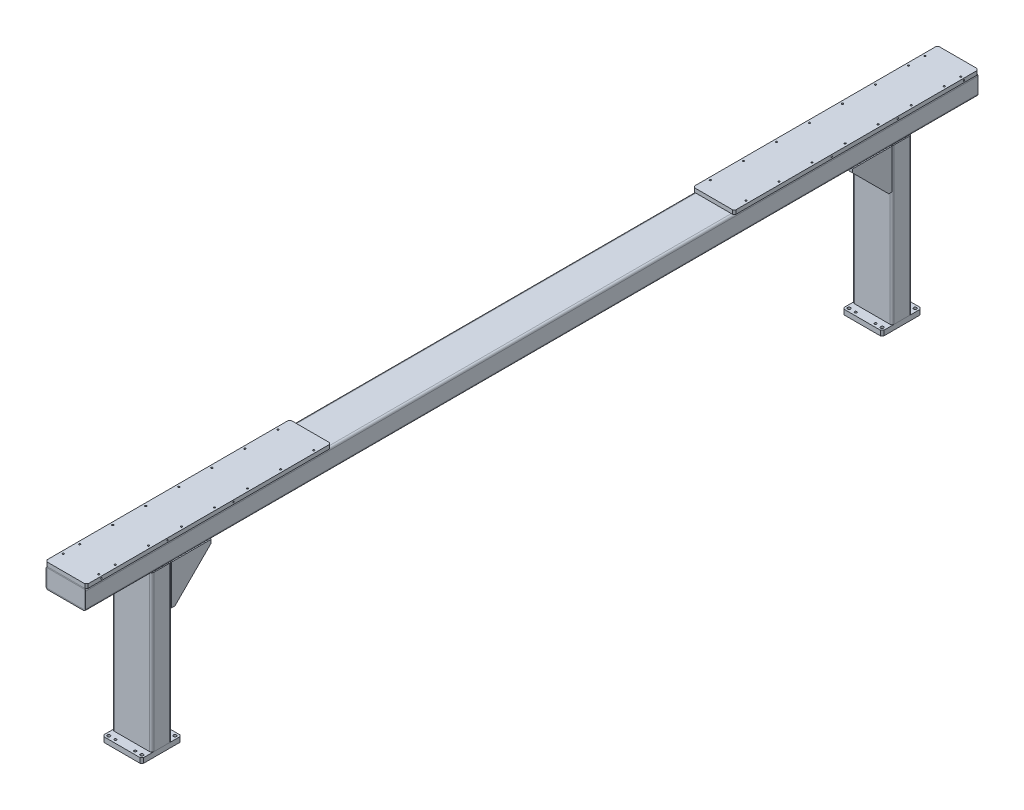
from build123d import *

# Parameters (mm, degrees)
F_120_X_60_X_3_2_1_DEPTH       = 500
F_120_X_60_X_3_2_1_2_DEPTH     = 500
F_120_X_60_X_3_2_2_DEPTH       = 2700
SKETCH_4_W                     = 125
SKETCH_4_H                     = 740
EXTRUDE_1_DEPTH                = 12
SKETCH_5_W                     = 120
SKETCH_5_H                     = 120
EXTRUDE_2_DEPTH                = 15
EXTRUDE_2_2_DEPTH              = 15
HOLE_WIZARD_9_0_9_1_AT_2_COUNT = 2
HOLE_WIZARD_9_0_9_1_AT_2_PITCH = 100
HOLE_WIZARD_9_0_9_1_AT_3_COUNT = 2
HOLE_WIZARD_9_0_9_1_AT_3_PITCH = 141.421356237
HOLE_WIZARD_9_0_9_1_AT_4_COUNT = 2
HOLE_WIZARD_9_0_9_1_AT_4_PITCH = 100
HOLE_WIZARD_9_0_9_1_AT_5_COUNT = 2
HOLE_WIZARD_9_0_9_1_AT_5_PITCH = 2342.135777448
HOLE_WIZARD_9_0_9_1_AT_6_COUNT = 2
HOLE_WIZARD_9_0_9_1_AT_6_PITCH = 2242.231031807
HOLE_WIZARD_9_0_9_1_AT_7_COUNT = 2
HOLE_WIZARD_9_0_9_1_AT_7_PITCH = 2240
HOLE_WIZARD_9_0_9_1_AT_8_COUNT = 2
HOLE_WIZARD_9_0_9_1_AT_8_PITCH = 2340
HOLE_WIZARD_M8_1_AT_2_COUNT    = 2
HOLE_WIZARD_M8_1_AT_2_PITCH    = 100
HOLE_WIZARD_M8_1_AT_3_COUNT    = 2
HOLE_WIZARD_M8_1_AT_3_PITCH    = 116.619037897
HOLE_WIZARD_M8_1_AT_4_COUNT    = 2
HOLE_WIZARD_M8_1_AT_4_PITCH    = 60
HOLE_WIZARD_M8_1_AT_5_COUNT    = 2
HOLE_WIZARD_M8_1_AT_5_PITCH    = 2140.84095626
HOLE_WIZARD_M8_1_AT_6_COUNT    = 2
HOLE_WIZARD_M8_1_AT_6_PITCH    = 2240.803427345
HOLE_WIZARD_M8_1_AT_7_COUNT    = 2
HOLE_WIZARD_M8_1_AT_7_PITCH    = 2240
HOLE_WIZARD_M8_1_AT_8_COUNT    = 2
HOLE_WIZARD_M8_1_AT_8_PITCH    = 2140
CHAMFER_1_SIZE                 = 5
HOLE_WIZARD_M6_1_AT_2_COUNT    = 2
HOLE_WIZARD_M6_1_AT_2_PITCH    = 108
HOLE_WIZARD_M6_1_AT_3_COUNT    = 2
HOLE_WIZARD_M6_1_AT_3_PITCH    = 147.186955944
HOLE_WIZARD_M6_1_AT_4_COUNT    = 2
HOLE_WIZARD_M6_1_AT_4_PITCH    = 227.297162323
HOLE_WIZARD_M6_1_AT_5_COUNT    = 2
HOLE_WIZARD_M6_1_AT_5_PITCH    = 318.847926134
HOLE_WIZARD_M6_1_AT_6_COUNT    = 2
HOLE_WIZARD_M6_1_AT_6_PITCH    = 414.323545071
HOLE_WIZARD_M6_1_AT_7_COUNT    = 2
HOLE_WIZARD_M6_1_AT_7_PITCH    = 511.531035227
HOLE_WIZARD_M6_1_AT_8_COUNT    = 2
HOLE_WIZARD_M6_1_AT_8_PITCH    = 100
HOLE_WIZARD_M6_1_AT_9_COUNT    = 2
HOLE_WIZARD_M6_1_AT_9_PITCH    = 200
HOLE_WIZARD_M6_1_AT_10_COUNT   = 2
HOLE_WIZARD_M6_1_AT_10_PITCH   = 300
HOLE_WIZARD_M6_1_AT_11_COUNT   = 2
HOLE_WIZARD_M6_1_AT_11_PITCH   = 400
HOLE_WIZARD_M6_1_AT_12_COUNT   = 2
HOLE_WIZARD_M6_1_AT_12_PITCH   = 500
HOLE_WIZARD_M6_1_AT_13_COUNT   = 2
HOLE_WIZARD_M6_1_AT_13_PITCH   = 650
HOLE_WIZARD_M6_1_AT_14_COUNT   = 2
HOLE_WIZARD_M6_1_AT_14_PITCH   = 658.911223155
HOLE_WIZARD_M6_1_AT_15_COUNT   = 2
HOLE_WIZARD_M6_1_AT_15_PITCH   = 600
HOLE_WIZARD_M6_1_AT_16_COUNT   = 2
HOLE_WIZARD_M6_1_AT_16_PITCH   = 609.642518202
CHAMFER_3_SIZE                 = 5
HOLE_WIZARD_M5_1_AT_2_COUNT    = 2
HOLE_WIZARD_M5_1_AT_2_PITCH    = 200
HOLE_WIZARD_M5_1_AT_3_COUNT    = 2
HOLE_WIZARD_M5_1_AT_3_PITCH    = 400
CHAMFER_4_SIZE                 = 5
SKETCH_32_W                    = 700
SKETCH_32_H                    = 15
EXTRUDE_3_DEPTH                = 7
EXTRUDE_3_2_DEPTH              = 7
HOLE_WIZARD_M4_3_AT_2_COUNT    = 2
HOLE_WIZARD_M4_3_AT_2_PITCH    = 60
HOLE_WIZARD_M4_3_AT_3_COUNT    = 2
HOLE_WIZARD_M4_3_AT_3_PITCH    = 120
HOLE_WIZARD_M4_3_AT_4_COUNT    = 2
HOLE_WIZARD_M4_3_AT_4_PITCH    = 180
HOLE_WIZARD_M4_3_AT_5_COUNT    = 2
HOLE_WIZARD_M4_3_AT_5_PITCH    = 240
HOLE_WIZARD_M4_3_AT_6_COUNT    = 2
HOLE_WIZARD_M4_3_AT_6_PITCH    = 300
HOLE_WIZARD_M4_3_AT_7_COUNT    = 2
HOLE_WIZARD_M4_3_AT_7_PITCH    = 360
HOLE_WIZARD_M4_3_AT_8_COUNT    = 2
HOLE_WIZARD_M4_3_AT_8_PITCH    = 420
HOLE_WIZARD_M4_3_AT_9_COUNT    = 2
HOLE_WIZARD_M4_3_AT_9_PITCH    = 480
HOLE_WIZARD_M4_3_AT_10_COUNT   = 2
HOLE_WIZARD_M4_3_AT_10_PITCH   = 540
HOLE_WIZARD_M4_3_AT_11_COUNT   = 2
HOLE_WIZARD_M4_3_AT_11_PITCH   = 600
HOLE_WIZARD_M4_3_AT_12_COUNT   = 2
HOLE_WIZARD_M4_3_AT_12_PITCH   = 660
HOLE_WIZARD_M4_3_AT_13_COUNT   = 2
HOLE_WIZARD_M4_3_AT_13_PITCH   = 1960
HOLE_WIZARD_M4_3_AT_14_COUNT   = 2
HOLE_WIZARD_M4_3_AT_14_PITCH   = 2020
HOLE_WIZARD_M4_3_AT_15_COUNT   = 2
HOLE_WIZARD_M4_3_AT_15_PITCH   = 2080
HOLE_WIZARD_M4_3_AT_16_COUNT   = 2
HOLE_WIZARD_M4_3_AT_16_PITCH   = 2140
HOLE_WIZARD_M4_3_AT_17_COUNT   = 2
HOLE_WIZARD_M4_3_AT_17_PITCH   = 2200
HOLE_WIZARD_M4_3_AT_18_COUNT   = 2
HOLE_WIZARD_M4_3_AT_18_PITCH   = 2260
HOLE_WIZARD_M4_3_AT_19_COUNT   = 2
HOLE_WIZARD_M4_3_AT_19_PITCH   = 2320
HOLE_WIZARD_M4_3_AT_20_COUNT   = 2
HOLE_WIZARD_M4_3_AT_20_PITCH   = 2380
HOLE_WIZARD_M4_3_AT_21_COUNT   = 2
HOLE_WIZARD_M4_3_AT_21_PITCH   = 2440
HOLE_WIZARD_M4_3_AT_22_COUNT   = 2
HOLE_WIZARD_M4_3_AT_22_PITCH   = 2500
HOLE_WIZARD_M4_3_AT_23_COUNT   = 2
HOLE_WIZARD_M4_3_AT_23_PITCH   = 2560
HOLE_WIZARD_M4_3_AT_24_COUNT   = 2
HOLE_WIZARD_M4_3_AT_24_PITCH   = 2620
HOLE_WIZARD_M4_4_AT_2_COUNT    = 2
HOLE_WIZARD_M4_4_AT_2_PITCH    = 690
HOLE_WIZARD_M4_4_AT_3_COUNT    = 2
HOLE_WIZARD_M4_4_AT_3_PITCH    = 1960
HOLE_WIZARD_M4_4_AT_4_COUNT    = 2
HOLE_WIZARD_M4_4_AT_4_PITCH    = 2650
EXTRUDE_4_DEPTH                = 5
EXTRUDE_5_DEPTH                = 10


with BuildPart() as part:
    # Sketch12 → 矩型管 120 X 60 X 3.2(1) (new body)
    with BuildSketch(Plane(origin=(0, 500, -1120), x_dir=(0, 0, -1), z_dir=(0, -1, 0))):
        with BuildLine():
            Line((-23.6, -60), (23.6, -60))
            ThreePointArc((23.6, -60), (28.1254834, -58.1254834), (30, -53.6))
            Line((30, -53.6), (30, 53.6))
            ThreePointArc((30, 53.6), (28.1254834, 58.1254834), (23.6, 60))
            Line((23.6, 60), (-23.6, 60))
            ThreePointArc((-23.6, 60), (-28.1254834, 58.1254834), (-30, 53.6))
            Line((-30, 53.6), (-30, -53.6))
            ThreePointArc((-30, -53.6), (-28.1254834, -58.1254834), (-23.6, -60))
        make_face()
        with BuildLine():
            Line((-23.6, -56.8), (23.6, -56.8))
            ThreePointArc((23.6, -56.8), (25.8627417, -55.8627417), (26.8, -53.6))
            Line((26.8, -53.6), (26.8, 53.6))
            ThreePointArc((26.8, 53.6), (25.8627417, 55.8627417), (23.6, 56.8))
            Line((23.6, 56.8), (-23.6, 56.8))
            ThreePointArc((-23.6, 56.8), (-25.8627417, 55.8627417), (-26.8, 53.6))
            Line((-26.8, 53.6), (-26.8, -53.6))
            ThreePointArc((-26.8, -53.6), (-25.8627417, -55.8627417), (-23.6, -56.8))
        make_face(mode=Mode.SUBTRACT)
    extrude(amount=F_120_X_60_X_3_2_1_DEPTH)

    # Weld Trim 1
    split(bisect_by=Plane.XZ.offset(-470), keep=Keep.TOP)


with BuildPart() as body_2:
    # Sketch12 on segment 2 (carried to segment 2) → 120 X 60 X 3.2_1 2 (new body)
    with BuildSketch(Plane(origin=(0, 500, 1120), x_dir=(0, 0, -1), z_dir=(0, -1, 0))):
        with BuildLine():
            Line((-23.6, -60), (23.6, -60))
            ThreePointArc((23.6, -60), (28.1254834, -58.1254834), (30, -53.6))
            Line((30, -53.6), (30, 53.6))
            ThreePointArc((30, 53.6), (28.1254834, 58.1254834), (23.6, 60))
            Line((23.6, 60), (-23.6, 60))
            ThreePointArc((-23.6, 60), (-28.1254834, 58.1254834), (-30, 53.6))
            Line((-30, 53.6), (-30, -53.6))
            ThreePointArc((-30, -53.6), (-28.1254834, -58.1254834), (-23.6, -60))
        make_face()
        with BuildLine():
            Line((-23.6, -56.8), (23.6, -56.8))
            ThreePointArc((23.6, -56.8), (25.8627417, -55.8627417), (26.8, -53.6))
            Line((26.8, -53.6), (26.8, 53.6))
            ThreePointArc((26.8, 53.6), (25.8627417, 55.8627417), (23.6, 56.8))
            Line((23.6, 56.8), (-23.6, 56.8))
            ThreePointArc((-23.6, 56.8), (-25.8627417, 55.8627417), (-26.8, 53.6))
            Line((-26.8, 53.6), (-26.8, -53.6))
            ThreePointArc((-26.8, -53.6), (-25.8627417, -55.8627417), (-23.6, -56.8))
        make_face(mode=Mode.SUBTRACT)
    extrude(amount=F_120_X_60_X_3_2_1_2_DEPTH)

    # Weld Trim 1
    split(bisect_by=Plane.XZ.offset(-470), keep=Keep.TOP)


with BuildPart() as body_3:
    # Sketch1 → 矩型管 120 X 60 X 3.2(2) (new body)
    with BuildSketch(Plane(origin=(0, 500, 1350), x_dir=(0, 1, 0), z_dir=(0, 0, -1))):
        with BuildLine():
            Line((-23.6, -60), (23.6, -60))
            ThreePointArc((23.6, -60), (28.1254834, -58.1254834), (30, -53.6))
            Line((30, -53.6), (30, 53.6))
            ThreePointArc((30, 53.6), (28.1254834, 58.1254834), (23.6, 60))
            Line((23.6, 60), (-23.6, 60))
            ThreePointArc((-23.6, 60), (-28.1254834, 58.1254834), (-30, 53.6))
            Line((-30, 53.6), (-30, -53.6))
            ThreePointArc((-30, -53.6), (-28.1254834, -58.1254834), (-23.6, -60))
        make_face()
        with BuildLine():
            Line((-23.6, -56.8), (23.6, -56.8))
            ThreePointArc((23.6, -56.8), (25.8627417, -55.8627417), (26.8, -53.6))
            Line((26.8, -53.6), (26.8, 53.6))
            ThreePointArc((26.8, 53.6), (25.8627417, 55.8627417), (23.6, 56.8))
            Line((23.6, 56.8), (-23.6, 56.8))
            ThreePointArc((-23.6, 56.8), (-25.8627417, 55.8627417), (-26.8, 53.6))
            Line((-26.8, 53.6), (-26.8, -53.6))
            ThreePointArc((-26.8, -53.6), (-25.8627417, -55.8627417), (-23.6, -56.8))
        make_face(mode=Mode.SUBTRACT)
    extrude(amount=F_120_X_60_X_3_2_2_DEPTH)


with BuildPart() as body_4:
    # 草图4 → 凸台-拉伸1 (new body)
    with BuildSketch(Plane(origin=(0, 530, 0), x_dir=(1, 0, 0), z_dir=(0, 1, 0))):
        with Locations((0, 980)):
            Rectangle(SKETCH_4_W, SKETCH_4_H)
    extrude(amount=EXTRUDE_1_DEPTH)

    # 草图25 → M6 螺纹孔1 (revolve, cut)
    with BuildSketch(Plane(origin=(54, 542, -654), x_dir=(0, 0, 1), z_dir=(1, 0, 0))):
        Polygon((0, 0), (0, 16.502151548), (2.5, 15), (2.5, 0), align=None)
    hole_wizard_m6_1 = revolve(axis=Axis((54, 548.35, -654), (0, -1, 0)), mode=Mode.SUBTRACT)

    # M6 螺纹孔1 at 2: M6 螺纹孔1 ×2
    with Locations(*[(-i * HOLE_WIZARD_M6_1_AT_2_PITCH, 0, 0) for i in range(1, HOLE_WIZARD_M6_1_AT_2_COUNT)]):
        add(hole_wizard_m6_1, mode=Mode.SUBTRACT)

    # M6 螺纹孔1 at 3: M6 螺纹孔1 ×2
    with Locations(*[Vector(-0.7337606740181704, 0, -0.679408031498304) * (i * HOLE_WIZARD_M6_1_AT_3_PITCH) for i in range(1, HOLE_WIZARD_M6_1_AT_3_COUNT)]):
        add(hole_wizard_m6_1, mode=Mode.SUBTRACT)

    # M6 螺纹孔1 at 4: M6 螺纹孔1 ×2
    with Locations(*[Vector(-0.47514891473488374, 0, -0.8799053976571926) * (i * HOLE_WIZARD_M6_1_AT_4_PITCH) for i in range(1, HOLE_WIZARD_M6_1_AT_4_COUNT)]):
        add(hole_wizard_m6_1, mode=Mode.SUBTRACT)

    # M6 螺纹孔1 at 5: M6 螺纹孔1 ×2
    with Locations(*[Vector(-0.3387194682727412, 0, -0.940887411868727) * (i * HOLE_WIZARD_M6_1_AT_5_PITCH) for i in range(1, HOLE_WIZARD_M6_1_AT_5_COUNT)]):
        add(hole_wizard_m6_1, mode=Mode.SUBTRACT)

    # M6 螺纹孔1 at 6: M6 螺纹孔1 ×2
    with Locations(*[Vector(-0.26066585229076417, 0, -0.9654290825583873) * (i * HOLE_WIZARD_M6_1_AT_6_PITCH) for i in range(1, HOLE_WIZARD_M6_1_AT_6_COUNT)]):
        add(hole_wizard_m6_1, mode=Mode.SUBTRACT)

    # M6 螺纹孔1 at 7: M6 螺纹孔1 ×2
    with Locations(*[Vector(-0.21113088466305252, 0, -0.9774577993659864) * (i * HOLE_WIZARD_M6_1_AT_7_PITCH) for i in range(1, HOLE_WIZARD_M6_1_AT_7_COUNT)]):
        add(hole_wizard_m6_1, mode=Mode.SUBTRACT)

    # M6 螺纹孔1 at 8: M6 螺纹孔1 ×2
    with Locations(*[(0, 0, -i * HOLE_WIZARD_M6_1_AT_8_PITCH) for i in range(1, HOLE_WIZARD_M6_1_AT_8_COUNT)]):
        add(hole_wizard_m6_1, mode=Mode.SUBTRACT)

    # M6 螺纹孔1 at 9: M6 螺纹孔1 ×2
    with Locations(*[(0, 0, -i * HOLE_WIZARD_M6_1_AT_9_PITCH) for i in range(1, HOLE_WIZARD_M6_1_AT_9_COUNT)]):
        add(hole_wizard_m6_1, mode=Mode.SUBTRACT)

    # M6 螺纹孔1 at 10: M6 螺纹孔1 ×2
    with Locations(*[(0, 0, -i * HOLE_WIZARD_M6_1_AT_10_PITCH) for i in range(1, HOLE_WIZARD_M6_1_AT_10_COUNT)]):
        add(hole_wizard_m6_1, mode=Mode.SUBTRACT)

    # M6 螺纹孔1 at 11: M6 螺纹孔1 ×2
    with Locations(*[(0, 0, -i * HOLE_WIZARD_M6_1_AT_11_PITCH) for i in range(1, HOLE_WIZARD_M6_1_AT_11_COUNT)]):
        add(hole_wizard_m6_1, mode=Mode.SUBTRACT)

    # M6 螺纹孔1 at 12: M6 螺纹孔1 ×2
    with Locations(*[(0, 0, -i * HOLE_WIZARD_M6_1_AT_12_PITCH) for i in range(1, HOLE_WIZARD_M6_1_AT_12_COUNT)]):
        add(hole_wizard_m6_1, mode=Mode.SUBTRACT)

    # M6 螺纹孔1 at 13: M6 螺纹孔1 ×2
    with Locations(*[(0, 0, -i * HOLE_WIZARD_M6_1_AT_13_PITCH) for i in range(1, HOLE_WIZARD_M6_1_AT_13_COUNT)]):
        add(hole_wizard_m6_1, mode=Mode.SUBTRACT)

    # M6 螺纹孔1 at 14: M6 螺纹孔1 ×2
    with Locations(*[Vector(-0.16390675436187938, 0, -0.9864758364372412) * (i * HOLE_WIZARD_M6_1_AT_14_PITCH) for i in range(1, HOLE_WIZARD_M6_1_AT_14_COUNT)]):
        add(hole_wizard_m6_1, mode=Mode.SUBTRACT)

    # M6 螺纹孔1 at 15: M6 螺纹孔1 ×2
    with Locations(*[(0, 0, -i * HOLE_WIZARD_M6_1_AT_15_PITCH) for i in range(1, HOLE_WIZARD_M6_1_AT_15_COUNT)]):
        add(hole_wizard_m6_1, mode=Mode.SUBTRACT)

    # M6 螺纹孔1 at 16: M6 螺纹孔1 ×2
    with Locations(*[Vector(-0.17715299831526468, 0, -0.9841833239736955) * (i * HOLE_WIZARD_M6_1_AT_16_PITCH) for i in range(1, HOLE_WIZARD_M6_1_AT_16_COUNT)]):
        add(hole_wizard_m6_1, mode=Mode.SUBTRACT)

    # 倒角3
    chamfer_3_edges = [body_4.edges().sort_by_distance(p)[0] for p in [
        (-62.5, 536, -610),
        (-62.5, 536, -1350),
        (62.5, 536, -1350),
        (62.5, 536, -610),
    ]]
    chamfer(chamfer_3_edges, length=CHAMFER_3_SIZE)

    # 草图27 → M5 螺纹孔1 (revolve, cut)
    with BuildSketch(Plane(origin=(62.5, 536, -905), x_dir=(0, 0, -1), z_dir=(0, 1, 0))):
        Polygon((0, 0), (0, 13.6618073), (2.1, 12.4), (2.1, 0), align=None)
    hole_wizard_m5_1 = revolve(axis=Axis((68.85, 536, -905), (-1, 0, 0)), mode=Mode.SUBTRACT)

    # M5 螺纹孔1 at 2: M5 螺纹孔1 ×2
    with Locations(*[(0, 0, -i * HOLE_WIZARD_M5_1_AT_2_PITCH) for i in range(1, HOLE_WIZARD_M5_1_AT_2_COUNT)]):
        add(hole_wizard_m5_1, mode=Mode.SUBTRACT)

    # M5 螺纹孔1 at 3: M5 螺纹孔1 ×2
    with Locations(*[(0, 0, -i * HOLE_WIZARD_M5_1_AT_3_PITCH) for i in range(1, HOLE_WIZARD_M5_1_AT_3_COUNT)]):
        add(hole_wizard_m5_1, mode=Mode.SUBTRACT)

    # 镜向1: M5 螺纹孔1 across plane
    add(hole_wizard_m5_1.mirror(Plane(origin=(0, 0, 0), x_dir=(0, 0, 1), z_dir=(1, 0, 0))), mode=Mode.SUBTRACT)

    # 镜向1 copy 1 sketch → 镜向1 copy 1 (revolve, cut)
    with BuildSketch(Plane(origin=(-62.5, 536, -1105), x_dir=(0, 0, -1), z_dir=(0, 1, 0))):
        Polygon((0, 0), (0, -13.6618073), (2.1, -12.4), (2.1, 0), align=None)
    revolve(axis=Axis((-68.85, 536, -1105), (-1, 0, 0)), mode=Mode.SUBTRACT)

    # 镜向1 copy 2 sketch → 镜向1 copy 2 (revolve, cut)
    with BuildSketch(Plane(origin=(-62.5, 536, -1305), x_dir=(0, 0, -1), z_dir=(0, 1, 0))):
        Polygon((0, 0), (0, -13.6618073), (2.1, -12.4), (2.1, 0), align=None)
    revolve(axis=Axis((-68.85, 536, -1305), (-1, 0, 0)), mode=Mode.SUBTRACT)


with BuildPart() as body_5:
    # 草图5 → 凸台-拉伸2 (new body)
    with BuildSketch(Plane.XZ):
        with Locations((0, 1120)):
            Rectangle(SKETCH_5_W, SKETCH_5_H)
    extrude(amount=EXTRUDE_2_DEPTH)


with BuildPart() as body_6:
    # 草图5 → Extrude 2 2 (new body)
    with BuildSketch(Plane.XZ):
        with Locations((0, -1120)):
            Rectangle(SKETCH_5_W, SKETCH_5_H)
    extrude(amount=EXTRUDE_2_2_DEPTH)

    # 草图15 → Ø9.0 (9) 直径孔1 (revolve, cut)
    with BuildSketch(Plane(origin=(-50, -15, -1170), x_dir=(0, 0, -1), z_dir=(1, 0, 0))):
        Polygon((0, 0), (0, 22.703872786), (4.5, 20), (4.5, 0), align=None)
    hole_wizard_9_0_9_1 = revolve(axis=Axis((-50, -21.35, -1170), (0, 1, 0)), mode=Mode.SUBTRACT)

    # Ø9.0 (9) 直径孔1 at 2: Ø9.0 (9) 直径孔1 ×2
    with Locations(*[(0, 0, i * HOLE_WIZARD_9_0_9_1_AT_2_PITCH) for i in range(1, HOLE_WIZARD_9_0_9_1_AT_2_COUNT)]):
        add(hole_wizard_9_0_9_1, mode=Mode.SUBTRACT)

    # Ø9.0 (9) 直径孔1 at 3: Ø9.0 (9) 直径孔1 ×2
    with Locations(*[Vector(0.7071067811865445, 0, 0.7071067811865507) * (i * HOLE_WIZARD_9_0_9_1_AT_3_PITCH) for i in range(1, HOLE_WIZARD_9_0_9_1_AT_3_COUNT)]):
        add(hole_wizard_9_0_9_1, mode=Mode.SUBTRACT)

    # Ø9.0 (9) 直径孔1 at 4: Ø9.0 (9) 直径孔1 ×2
    with Locations(*[(i * HOLE_WIZARD_9_0_9_1_AT_4_PITCH, 0, 0) for i in range(1, HOLE_WIZARD_9_0_9_1_AT_4_COUNT)]):
        add(hole_wizard_9_0_9_1, mode=Mode.SUBTRACT)

    # 草图13 → M8 螺纹孔1 (revolve, cut)
    with BuildSketch(Plane(origin=(-30, 0, -1070), x_dir=(0, 0, 1), z_dir=(1, 0, 0))):
        Polygon((0, 0), (0, 24.292926105), (3.4, 22.25), (3.4, 0), align=None)
    hole_wizard_m8_1 = revolve(axis=Axis((-30, 6.35, -1070), (0, -1, 0)), mode=Mode.SUBTRACT)

    # M8 螺纹孔1 at 2: M8 螺纹孔1 ×2
    with Locations(*[(0, 0, -i * HOLE_WIZARD_M8_1_AT_2_PITCH) for i in range(1, HOLE_WIZARD_M8_1_AT_2_COUNT)]):
        add(hole_wizard_m8_1, mode=Mode.SUBTRACT)

    # M8 螺纹孔1 at 3: M8 螺纹孔1 ×2
    with Locations(*[Vector(0.5144957554275295, 0, -0.8574929257125425) * (i * HOLE_WIZARD_M8_1_AT_3_PITCH) for i in range(1, HOLE_WIZARD_M8_1_AT_3_COUNT)]):
        add(hole_wizard_m8_1, mode=Mode.SUBTRACT)

    # M8 螺纹孔1 at 4: M8 螺纹孔1 ×2
    with Locations(*[(i * HOLE_WIZARD_M8_1_AT_4_PITCH, 0, 0) for i in range(1, HOLE_WIZARD_M8_1_AT_4_COUNT)]):
        add(hole_wizard_m8_1, mode=Mode.SUBTRACT)

    # 倒角4
    chamfer_4_edges = [body_6.edges().sort_by_distance(p)[0] for p in [
        (-60, -7.5, -1180),
        (-60, -7.5, -1060),
        (60, -7.5, -1060),
        (60, -7.5, -1180),
    ]]
    chamfer(chamfer_4_edges, length=CHAMFER_4_SIZE)


with BuildPart() as body_5_1:
    add(body_5.part)

    # Ø9.0 (9) 直径孔1 at 5: Ø9.0 (9) 直径孔1 ×2
    with Locations(*[Vector(0.04269607294457472, 0, 0.9990881069030457) * (i * HOLE_WIZARD_9_0_9_1_AT_5_PITCH) for i in range(1, HOLE_WIZARD_9_0_9_1_AT_5_COUNT)]):
        add(hole_wizard_9_0_9_1, mode=Mode.SUBTRACT)

    # Ø9.0 (9) 直径孔1 at 6: Ø9.0 (9) 直径孔1 ×2
    with Locations(*[Vector(0.044598437262458705, 0, 0.999004994679079) * (i * HOLE_WIZARD_9_0_9_1_AT_6_PITCH) for i in range(1, HOLE_WIZARD_9_0_9_1_AT_6_COUNT)]):
        add(hole_wizard_9_0_9_1, mode=Mode.SUBTRACT)

    # Ø9.0 (9) 直径孔1 at 7: Ø9.0 (9) 直径孔1 ×2
    with Locations(*[(0, 0, i * HOLE_WIZARD_9_0_9_1_AT_7_PITCH) for i in range(1, HOLE_WIZARD_9_0_9_1_AT_7_COUNT)]):
        add(hole_wizard_9_0_9_1, mode=Mode.SUBTRACT)

    # Ø9.0 (9) 直径孔1 at 8: Ø9.0 (9) 直径孔1 ×2
    with Locations(*[(0, 0, i * HOLE_WIZARD_9_0_9_1_AT_8_PITCH) for i in range(1, HOLE_WIZARD_9_0_9_1_AT_8_COUNT)]):
        add(hole_wizard_9_0_9_1, mode=Mode.SUBTRACT)

    # M8 螺纹孔1 at 5: M8 螺纹孔1 ×2
    with Locations(*[Vector(0.028026369649066126, 0, 0.999607184150001) * (i * HOLE_WIZARD_M8_1_AT_5_PITCH) for i in range(1, HOLE_WIZARD_M8_1_AT_5_COUNT)]):
        add(hole_wizard_m8_1, mode=Mode.SUBTRACT)

    # M8 螺纹孔1 at 6: M8 螺纹孔1 ×2
    with Locations(*[Vector(0.02677611041995684, 0, 0.9996414556783739) * (i * HOLE_WIZARD_M8_1_AT_6_PITCH) for i in range(1, HOLE_WIZARD_M8_1_AT_6_COUNT)]):
        add(hole_wizard_m8_1, mode=Mode.SUBTRACT)

    # M8 螺纹孔1 at 7: M8 螺纹孔1 ×2
    with Locations(*[(0, 0, i * HOLE_WIZARD_M8_1_AT_7_PITCH) for i in range(1, HOLE_WIZARD_M8_1_AT_7_COUNT)]):
        add(hole_wizard_m8_1, mode=Mode.SUBTRACT)

    # M8 螺纹孔1 at 8: M8 螺纹孔1 ×2
    with Locations(*[(0, 0, i * HOLE_WIZARD_M8_1_AT_8_PITCH) for i in range(1, HOLE_WIZARD_M8_1_AT_8_COUNT)]):
        add(hole_wizard_m8_1, mode=Mode.SUBTRACT)

    # 倒角1
    chamfer_1_edges = [body_5_1.edges().sort_by_distance(p)[0] for p in [
        (-60, -7.5, 1180),
        (60, -7.5, 1180),
        (60, -7.5, 1060),
        (-60, -7.5, 1060),
    ]]
    chamfer(chamfer_1_edges, length=CHAMFER_1_SIZE)


with BuildPart() as body_7:
    # 镜向3: mirrored copy
    add(body_4.part.mirror(Plane.XY))


with BuildPart() as body_8:
    # 草图32 → 凸台-拉伸3 (new body)
    with BuildSketch(Plane.ZY.offset(60)):
        with Locations((-980, 489.5)):
            Rectangle(SKETCH_32_W, SKETCH_32_H)
    extrude(amount=EXTRUDE_3_DEPTH)


with BuildPart() as body_9:
    # 草图32 → Extrude 3 2 (new body)
    with BuildSketch(Plane.ZY.offset(60)):
        with Locations((980, 489.5)):
            Rectangle(SKETCH_32_W, SKETCH_32_H)
    extrude(amount=EXTRUDE_3_2_DEPTH)


with BuildPart() as hole_wizard_m4_3_tool:
    # 草图35 → M4 螺纹孔3 (revolve)
    with BuildSketch(Plane(origin=(-67, 489.5, -1310), x_dir=(0, 0, 1), z_dir=(0, 1, 0))):
        Polygon((0, 0), (0, 11.091420021), (1.65, 10.1), (1.65, 0), align=None)
    hole_wizard_m4_3 = revolve(axis=Axis((-73.35, 489.5, -1310), (1, 0, 0)))


with BuildPart() as body_3_1:
    add(body_3.part)

    # M4 螺纹孔3: cut by hole_wizard_m4_3_tool
    add(hole_wizard_m4_3_tool.part, mode=Mode.SUBTRACT)


with BuildPart() as body_8_1:
    add(body_8.part)

    # M4 螺纹孔3: cut by hole_wizard_m4_3_tool
    add(hole_wizard_m4_3_tool.part, mode=Mode.SUBTRACT)


with BuildPart() as hole_wizard_m4_3_at_2_tool:
    # M4 螺纹孔3 at 2: M4 螺纹孔3 ×2
    with Locations(*[(0, 0, i * HOLE_WIZARD_M4_3_AT_2_PITCH) for i in range(1, HOLE_WIZARD_M4_3_AT_2_COUNT)]):
        add(hole_wizard_m4_3)


with BuildPart() as body_3_2:
    add(body_3_1.part)

    # M4 螺纹孔3 at 2: cut by hole_wizard_m4_3_at_2_tool
    add(hole_wizard_m4_3_at_2_tool.part, mode=Mode.SUBTRACT)


with BuildPart() as body_8_2:
    add(body_8_1.part)

    # M4 螺纹孔3 at 2: cut by hole_wizard_m4_3_at_2_tool
    add(hole_wizard_m4_3_at_2_tool.part, mode=Mode.SUBTRACT)


with BuildPart() as hole_wizard_m4_3_at_3_tool:
    # M4 螺纹孔3 at 3: M4 螺纹孔3 ×2
    with Locations(*[(0, 0, i * HOLE_WIZARD_M4_3_AT_3_PITCH) for i in range(1, HOLE_WIZARD_M4_3_AT_3_COUNT)]):
        add(hole_wizard_m4_3)


with BuildPart() as body_3_3:
    add(body_3_2.part)

    # M4 螺纹孔3 at 3: cut by hole_wizard_m4_3_at_3_tool
    add(hole_wizard_m4_3_at_3_tool.part, mode=Mode.SUBTRACT)


with BuildPart() as body_8_3:
    add(body_8_2.part)

    # M4 螺纹孔3 at 3: cut by hole_wizard_m4_3_at_3_tool
    add(hole_wizard_m4_3_at_3_tool.part, mode=Mode.SUBTRACT)


with BuildPart() as hole_wizard_m4_3_at_4_tool:
    # M4 螺纹孔3 at 4: M4 螺纹孔3 ×2
    with Locations(*[(0, 0, i * HOLE_WIZARD_M4_3_AT_4_PITCH) for i in range(1, HOLE_WIZARD_M4_3_AT_4_COUNT)]):
        add(hole_wizard_m4_3)


with BuildPart() as body_3_4:
    add(body_3_3.part)

    # M4 螺纹孔3 at 4: cut by hole_wizard_m4_3_at_4_tool
    add(hole_wizard_m4_3_at_4_tool.part, mode=Mode.SUBTRACT)


with BuildPart() as body_8_4:
    add(body_8_3.part)

    # M4 螺纹孔3 at 4: cut by hole_wizard_m4_3_at_4_tool
    add(hole_wizard_m4_3_at_4_tool.part, mode=Mode.SUBTRACT)


with BuildPart() as hole_wizard_m4_3_at_5_tool:
    # M4 螺纹孔3 at 5: M4 螺纹孔3 ×2
    with Locations(*[(0, 0, i * HOLE_WIZARD_M4_3_AT_5_PITCH) for i in range(1, HOLE_WIZARD_M4_3_AT_5_COUNT)]):
        add(hole_wizard_m4_3)


with BuildPart() as body_3_5:
    add(body_3_4.part)

    # M4 螺纹孔3 at 5: cut by hole_wizard_m4_3_at_5_tool
    add(hole_wizard_m4_3_at_5_tool.part, mode=Mode.SUBTRACT)


with BuildPart() as body_8_5:
    add(body_8_4.part)

    # M4 螺纹孔3 at 5: cut by hole_wizard_m4_3_at_5_tool
    add(hole_wizard_m4_3_at_5_tool.part, mode=Mode.SUBTRACT)


with BuildPart() as hole_wizard_m4_3_at_6_tool:
    # M4 螺纹孔3 at 6: M4 螺纹孔3 ×2
    with Locations(*[(0, 0, i * HOLE_WIZARD_M4_3_AT_6_PITCH) for i in range(1, HOLE_WIZARD_M4_3_AT_6_COUNT)]):
        add(hole_wizard_m4_3)


with BuildPart() as body_3_6:
    add(body_3_5.part)

    # M4 螺纹孔3 at 6: cut by hole_wizard_m4_3_at_6_tool
    add(hole_wizard_m4_3_at_6_tool.part, mode=Mode.SUBTRACT)


with BuildPart() as body_8_6:
    add(body_8_5.part)

    # M4 螺纹孔3 at 6: cut by hole_wizard_m4_3_at_6_tool
    add(hole_wizard_m4_3_at_6_tool.part, mode=Mode.SUBTRACT)


with BuildPart() as hole_wizard_m4_3_at_7_tool:
    # M4 螺纹孔3 at 7: M4 螺纹孔3 ×2
    with Locations(*[(0, 0, i * HOLE_WIZARD_M4_3_AT_7_PITCH) for i in range(1, HOLE_WIZARD_M4_3_AT_7_COUNT)]):
        add(hole_wizard_m4_3)


with BuildPart() as body_3_7:
    add(body_3_6.part)

    # M4 螺纹孔3 at 7: cut by hole_wizard_m4_3_at_7_tool
    add(hole_wizard_m4_3_at_7_tool.part, mode=Mode.SUBTRACT)


with BuildPart() as body_8_7:
    add(body_8_6.part)

    # M4 螺纹孔3 at 7: cut by hole_wizard_m4_3_at_7_tool
    add(hole_wizard_m4_3_at_7_tool.part, mode=Mode.SUBTRACT)


with BuildPart() as hole_wizard_m4_3_at_8_tool:
    # M4 螺纹孔3 at 8: M4 螺纹孔3 ×2
    with Locations(*[(0, 0, i * HOLE_WIZARD_M4_3_AT_8_PITCH) for i in range(1, HOLE_WIZARD_M4_3_AT_8_COUNT)]):
        add(hole_wizard_m4_3)


with BuildPart() as body_3_8:
    add(body_3_7.part)

    # M4 螺纹孔3 at 8: cut by hole_wizard_m4_3_at_8_tool
    add(hole_wizard_m4_3_at_8_tool.part, mode=Mode.SUBTRACT)


with BuildPart() as body_8_8:
    add(body_8_7.part)

    # M4 螺纹孔3 at 8: cut by hole_wizard_m4_3_at_8_tool
    add(hole_wizard_m4_3_at_8_tool.part, mode=Mode.SUBTRACT)


with BuildPart() as hole_wizard_m4_3_at_9_tool:
    # M4 螺纹孔3 at 9: M4 螺纹孔3 ×2
    with Locations(*[(0, 0, i * HOLE_WIZARD_M4_3_AT_9_PITCH) for i in range(1, HOLE_WIZARD_M4_3_AT_9_COUNT)]):
        add(hole_wizard_m4_3)


with BuildPart() as body_3_9:
    add(body_3_8.part)

    # M4 螺纹孔3 at 9: cut by hole_wizard_m4_3_at_9_tool
    add(hole_wizard_m4_3_at_9_tool.part, mode=Mode.SUBTRACT)


with BuildPart() as body_8_9:
    add(body_8_8.part)

    # M4 螺纹孔3 at 9: cut by hole_wizard_m4_3_at_9_tool
    add(hole_wizard_m4_3_at_9_tool.part, mode=Mode.SUBTRACT)


with BuildPart() as hole_wizard_m4_3_at_10_tool:
    # M4 螺纹孔3 at 10: M4 螺纹孔3 ×2
    with Locations(*[(0, 0, i * HOLE_WIZARD_M4_3_AT_10_PITCH) for i in range(1, HOLE_WIZARD_M4_3_AT_10_COUNT)]):
        add(hole_wizard_m4_3)


with BuildPart() as body_3_10:
    add(body_3_9.part)

    # M4 螺纹孔3 at 10: cut by hole_wizard_m4_3_at_10_tool
    add(hole_wizard_m4_3_at_10_tool.part, mode=Mode.SUBTRACT)


with BuildPart() as body_8_10:
    add(body_8_9.part)

    # M4 螺纹孔3 at 10: cut by hole_wizard_m4_3_at_10_tool
    add(hole_wizard_m4_3_at_10_tool.part, mode=Mode.SUBTRACT)


with BuildPart() as hole_wizard_m4_3_at_11_tool:
    # M4 螺纹孔3 at 11: M4 螺纹孔3 ×2
    with Locations(*[(0, 0, i * HOLE_WIZARD_M4_3_AT_11_PITCH) for i in range(1, HOLE_WIZARD_M4_3_AT_11_COUNT)]):
        add(hole_wizard_m4_3)


with BuildPart() as body_3_11:
    add(body_3_10.part)

    # M4 螺纹孔3 at 11: cut by hole_wizard_m4_3_at_11_tool
    add(hole_wizard_m4_3_at_11_tool.part, mode=Mode.SUBTRACT)


with BuildPart() as body_8_11:
    add(body_8_10.part)

    # M4 螺纹孔3 at 11: cut by hole_wizard_m4_3_at_11_tool
    add(hole_wizard_m4_3_at_11_tool.part, mode=Mode.SUBTRACT)


with BuildPart() as hole_wizard_m4_3_at_12_tool:
    # M4 螺纹孔3 at 12: M4 螺纹孔3 ×2
    with Locations(*[(0, 0, i * HOLE_WIZARD_M4_3_AT_12_PITCH) for i in range(1, HOLE_WIZARD_M4_3_AT_12_COUNT)]):
        add(hole_wizard_m4_3)


with BuildPart() as body_3_12:
    add(body_3_11.part)

    # M4 螺纹孔3 at 12: cut by hole_wizard_m4_3_at_12_tool
    add(hole_wizard_m4_3_at_12_tool.part, mode=Mode.SUBTRACT)


with BuildPart() as body_8_12:
    add(body_8_11.part)

    # M4 螺纹孔3 at 12: cut by hole_wizard_m4_3_at_12_tool
    add(hole_wizard_m4_3_at_12_tool.part, mode=Mode.SUBTRACT)


with BuildPart() as hole_wizard_m4_3_at_13_tool:
    # M4 螺纹孔3 at 13: M4 螺纹孔3 ×2
    with Locations(*[(0, 0, i * HOLE_WIZARD_M4_3_AT_13_PITCH) for i in range(1, HOLE_WIZARD_M4_3_AT_13_COUNT)]):
        add(hole_wizard_m4_3)


with BuildPart() as body_3_13:
    add(body_3_12.part)

    # M4 螺纹孔3 at 13: cut by hole_wizard_m4_3_at_13_tool
    add(hole_wizard_m4_3_at_13_tool.part, mode=Mode.SUBTRACT)


with BuildPart() as body_9_1:
    add(body_9.part)

    # M4 螺纹孔3 at 13: cut by hole_wizard_m4_3_at_13_tool
    add(hole_wizard_m4_3_at_13_tool.part, mode=Mode.SUBTRACT)


with BuildPart() as hole_wizard_m4_3_at_14_tool:
    # M4 螺纹孔3 at 14: M4 螺纹孔3 ×2
    with Locations(*[(0, 0, i * HOLE_WIZARD_M4_3_AT_14_PITCH) for i in range(1, HOLE_WIZARD_M4_3_AT_14_COUNT)]):
        add(hole_wizard_m4_3)


with BuildPart() as body_3_14:
    add(body_3_13.part)

    # M4 螺纹孔3 at 14: cut by hole_wizard_m4_3_at_14_tool
    add(hole_wizard_m4_3_at_14_tool.part, mode=Mode.SUBTRACT)


with BuildPart() as body_9_2:
    add(body_9_1.part)

    # M4 螺纹孔3 at 14: cut by hole_wizard_m4_3_at_14_tool
    add(hole_wizard_m4_3_at_14_tool.part, mode=Mode.SUBTRACT)


with BuildPart() as hole_wizard_m4_3_at_15_tool:
    # M4 螺纹孔3 at 15: M4 螺纹孔3 ×2
    with Locations(*[(0, 0, i * HOLE_WIZARD_M4_3_AT_15_PITCH) for i in range(1, HOLE_WIZARD_M4_3_AT_15_COUNT)]):
        add(hole_wizard_m4_3)


with BuildPart() as body_3_15:
    add(body_3_14.part)

    # M4 螺纹孔3 at 15: cut by hole_wizard_m4_3_at_15_tool
    add(hole_wizard_m4_3_at_15_tool.part, mode=Mode.SUBTRACT)


with BuildPart() as body_9_3:
    add(body_9_2.part)

    # M4 螺纹孔3 at 15: cut by hole_wizard_m4_3_at_15_tool
    add(hole_wizard_m4_3_at_15_tool.part, mode=Mode.SUBTRACT)


with BuildPart() as hole_wizard_m4_3_at_16_tool:
    # M4 螺纹孔3 at 16: M4 螺纹孔3 ×2
    with Locations(*[(0, 0, i * HOLE_WIZARD_M4_3_AT_16_PITCH) for i in range(1, HOLE_WIZARD_M4_3_AT_16_COUNT)]):
        add(hole_wizard_m4_3)


with BuildPart() as body_3_16:
    add(body_3_15.part)

    # M4 螺纹孔3 at 16: cut by hole_wizard_m4_3_at_16_tool
    add(hole_wizard_m4_3_at_16_tool.part, mode=Mode.SUBTRACT)


with BuildPart() as body_9_4:
    add(body_9_3.part)

    # M4 螺纹孔3 at 16: cut by hole_wizard_m4_3_at_16_tool
    add(hole_wizard_m4_3_at_16_tool.part, mode=Mode.SUBTRACT)


with BuildPart() as hole_wizard_m4_3_at_17_tool:
    # M4 螺纹孔3 at 17: M4 螺纹孔3 ×2
    with Locations(*[(0, 0, i * HOLE_WIZARD_M4_3_AT_17_PITCH) for i in range(1, HOLE_WIZARD_M4_3_AT_17_COUNT)]):
        add(hole_wizard_m4_3)


with BuildPart() as body_3_17:
    add(body_3_16.part)

    # M4 螺纹孔3 at 17: cut by hole_wizard_m4_3_at_17_tool
    add(hole_wizard_m4_3_at_17_tool.part, mode=Mode.SUBTRACT)


with BuildPart() as body_9_5:
    add(body_9_4.part)

    # M4 螺纹孔3 at 17: cut by hole_wizard_m4_3_at_17_tool
    add(hole_wizard_m4_3_at_17_tool.part, mode=Mode.SUBTRACT)


with BuildPart() as hole_wizard_m4_3_at_18_tool:
    # M4 螺纹孔3 at 18: M4 螺纹孔3 ×2
    with Locations(*[(0, 0, i * HOLE_WIZARD_M4_3_AT_18_PITCH) for i in range(1, HOLE_WIZARD_M4_3_AT_18_COUNT)]):
        add(hole_wizard_m4_3)


with BuildPart() as body_3_18:
    add(body_3_17.part)

    # M4 螺纹孔3 at 18: cut by hole_wizard_m4_3_at_18_tool
    add(hole_wizard_m4_3_at_18_tool.part, mode=Mode.SUBTRACT)


with BuildPart() as body_9_6:
    add(body_9_5.part)

    # M4 螺纹孔3 at 18: cut by hole_wizard_m4_3_at_18_tool
    add(hole_wizard_m4_3_at_18_tool.part, mode=Mode.SUBTRACT)


with BuildPart() as hole_wizard_m4_3_at_19_tool:
    # M4 螺纹孔3 at 19: M4 螺纹孔3 ×2
    with Locations(*[(0, 0, i * HOLE_WIZARD_M4_3_AT_19_PITCH) for i in range(1, HOLE_WIZARD_M4_3_AT_19_COUNT)]):
        add(hole_wizard_m4_3)


with BuildPart() as body_3_19:
    add(body_3_18.part)

    # M4 螺纹孔3 at 19: cut by hole_wizard_m4_3_at_19_tool
    add(hole_wizard_m4_3_at_19_tool.part, mode=Mode.SUBTRACT)


with BuildPart() as body_9_7:
    add(body_9_6.part)

    # M4 螺纹孔3 at 19: cut by hole_wizard_m4_3_at_19_tool
    add(hole_wizard_m4_3_at_19_tool.part, mode=Mode.SUBTRACT)


with BuildPart() as hole_wizard_m4_3_at_20_tool:
    # M4 螺纹孔3 at 20: M4 螺纹孔3 ×2
    with Locations(*[(0, 0, i * HOLE_WIZARD_M4_3_AT_20_PITCH) for i in range(1, HOLE_WIZARD_M4_3_AT_20_COUNT)]):
        add(hole_wizard_m4_3)


with BuildPart() as body_3_20:
    add(body_3_19.part)

    # M4 螺纹孔3 at 20: cut by hole_wizard_m4_3_at_20_tool
    add(hole_wizard_m4_3_at_20_tool.part, mode=Mode.SUBTRACT)


with BuildPart() as body_9_8:
    add(body_9_7.part)

    # M4 螺纹孔3 at 20: cut by hole_wizard_m4_3_at_20_tool
    add(hole_wizard_m4_3_at_20_tool.part, mode=Mode.SUBTRACT)


with BuildPart() as hole_wizard_m4_3_at_21_tool:
    # M4 螺纹孔3 at 21: M4 螺纹孔3 ×2
    with Locations(*[(0, 0, i * HOLE_WIZARD_M4_3_AT_21_PITCH) for i in range(1, HOLE_WIZARD_M4_3_AT_21_COUNT)]):
        add(hole_wizard_m4_3)


with BuildPart() as body_3_21:
    add(body_3_20.part)

    # M4 螺纹孔3 at 21: cut by hole_wizard_m4_3_at_21_tool
    add(hole_wizard_m4_3_at_21_tool.part, mode=Mode.SUBTRACT)


with BuildPart() as body_9_9:
    add(body_9_8.part)

    # M4 螺纹孔3 at 21: cut by hole_wizard_m4_3_at_21_tool
    add(hole_wizard_m4_3_at_21_tool.part, mode=Mode.SUBTRACT)


with BuildPart() as hole_wizard_m4_3_at_22_tool:
    # M4 螺纹孔3 at 22: M4 螺纹孔3 ×2
    with Locations(*[(0, 0, i * HOLE_WIZARD_M4_3_AT_22_PITCH) for i in range(1, HOLE_WIZARD_M4_3_AT_22_COUNT)]):
        add(hole_wizard_m4_3)


with BuildPart() as body_3_22:
    add(body_3_21.part)

    # M4 螺纹孔3 at 22: cut by hole_wizard_m4_3_at_22_tool
    add(hole_wizard_m4_3_at_22_tool.part, mode=Mode.SUBTRACT)


with BuildPart() as body_9_10:
    add(body_9_9.part)

    # M4 螺纹孔3 at 22: cut by hole_wizard_m4_3_at_22_tool
    add(hole_wizard_m4_3_at_22_tool.part, mode=Mode.SUBTRACT)


with BuildPart() as hole_wizard_m4_3_at_23_tool:
    # M4 螺纹孔3 at 23: M4 螺纹孔3 ×2
    with Locations(*[(0, 0, i * HOLE_WIZARD_M4_3_AT_23_PITCH) for i in range(1, HOLE_WIZARD_M4_3_AT_23_COUNT)]):
        add(hole_wizard_m4_3)


with BuildPart() as body_3_23:
    add(body_3_22.part)

    # M4 螺纹孔3 at 23: cut by hole_wizard_m4_3_at_23_tool
    add(hole_wizard_m4_3_at_23_tool.part, mode=Mode.SUBTRACT)


with BuildPart() as body_9_11:
    add(body_9_10.part)

    # M4 螺纹孔3 at 23: cut by hole_wizard_m4_3_at_23_tool
    add(hole_wizard_m4_3_at_23_tool.part, mode=Mode.SUBTRACT)


with BuildPart() as hole_wizard_m4_3_at_24_tool:
    # M4 螺纹孔3 at 24: M4 螺纹孔3 ×2
    with Locations(*[(0, 0, i * HOLE_WIZARD_M4_3_AT_24_PITCH) for i in range(1, HOLE_WIZARD_M4_3_AT_24_COUNT)]):
        add(hole_wizard_m4_3)


with BuildPart() as body_3_24:
    add(body_3_23.part)

    # M4 螺纹孔3 at 24: cut by hole_wizard_m4_3_at_24_tool
    add(hole_wizard_m4_3_at_24_tool.part, mode=Mode.SUBTRACT)


with BuildPart() as body_9_12:
    add(body_9_11.part)

    # M4 螺纹孔3 at 24: cut by hole_wizard_m4_3_at_24_tool
    add(hole_wizard_m4_3_at_24_tool.part, mode=Mode.SUBTRACT)


with BuildPart() as hole_wizard_m4_4_tool:
    # 草图38 → M4 螺纹孔4 (revolve)
    with BuildSketch(Plane(origin=(-67, 489.5, -1325), x_dir=(0, 0, 1), z_dir=(0, 1, 0))):
        Polygon((0, 0), (0, 11.091420021), (1.65, 10.1), (1.65, 0), align=None)
    hole_wizard_m4_4 = revolve(axis=Axis((-73.35, 489.5, -1325), (1, 0, 0)))


with BuildPart() as body_3_25:
    add(body_3_24.part)

    # M4 螺纹孔4: cut by hole_wizard_m4_4_tool
    add(hole_wizard_m4_4_tool.part, mode=Mode.SUBTRACT)


with BuildPart() as body_8_13:
    add(body_8_12.part)

    # M4 螺纹孔4: cut by hole_wizard_m4_4_tool
    add(hole_wizard_m4_4_tool.part, mode=Mode.SUBTRACT)


with BuildPart() as hole_wizard_m4_4_at_2_tool:
    # M4 螺纹孔4 at 2: M4 螺纹孔4 ×2
    with Locations(*[(0, 0, i * HOLE_WIZARD_M4_4_AT_2_PITCH) for i in range(1, HOLE_WIZARD_M4_4_AT_2_COUNT)]):
        add(hole_wizard_m4_4)


with BuildPart() as body_3_26:
    add(body_3_25.part)

    # M4 螺纹孔4 at 2: cut by hole_wizard_m4_4_at_2_tool
    add(hole_wizard_m4_4_at_2_tool.part, mode=Mode.SUBTRACT)


with BuildPart() as body_8_14:
    add(body_8_13.part)

    # M4 螺纹孔4 at 2: cut by hole_wizard_m4_4_at_2_tool
    add(hole_wizard_m4_4_at_2_tool.part, mode=Mode.SUBTRACT)


with BuildPart() as hole_wizard_m4_4_at_3_tool:
    # M4 螺纹孔4 at 3: M4 螺纹孔4 ×2
    with Locations(*[(0, 0, i * HOLE_WIZARD_M4_4_AT_3_PITCH) for i in range(1, HOLE_WIZARD_M4_4_AT_3_COUNT)]):
        add(hole_wizard_m4_4)


with BuildPart() as body_3_27:
    add(body_3_26.part)

    # M4 螺纹孔4 at 3: cut by hole_wizard_m4_4_at_3_tool
    add(hole_wizard_m4_4_at_3_tool.part, mode=Mode.SUBTRACT)


with BuildPart() as body_9_13:
    add(body_9_12.part)

    # M4 螺纹孔4 at 3: cut by hole_wizard_m4_4_at_3_tool
    add(hole_wizard_m4_4_at_3_tool.part, mode=Mode.SUBTRACT)


with BuildPart() as hole_wizard_m4_4_at_4_tool:
    # M4 螺纹孔4 at 4: M4 螺纹孔4 ×2
    with Locations(*[(0, 0, i * HOLE_WIZARD_M4_4_AT_4_PITCH) for i in range(1, HOLE_WIZARD_M4_4_AT_4_COUNT)]):
        add(hole_wizard_m4_4)


with BuildPart() as body_3_28:
    add(body_3_27.part)

    # M4 螺纹孔4 at 4: cut by hole_wizard_m4_4_at_4_tool
    add(hole_wizard_m4_4_at_4_tool.part, mode=Mode.SUBTRACT)


with BuildPart() as body_9_14:
    add(body_9_13.part)

    # M4 螺纹孔4 at 4: cut by hole_wizard_m4_4_at_4_tool
    add(hole_wizard_m4_4_at_4_tool.part, mode=Mode.SUBTRACT)


with BuildPart() as body_10:
    # 草图39 → 凸台-拉伸4 (new body)
    with BuildSketch(Plane(origin=(0, 0, -1350), x_dir=(-1, 0, 0), z_dir=(0, 0, -1))):
        with BuildLine():
            Line((56.8, 476.4), (56.8, 523.6))
            ThreePointArc((56.8, 523.6), (55.8627417, 525.8627417), (53.6, 526.8))
            Line((53.6, 526.8), (-53.6, 526.8))
            ThreePointArc((-53.6, 526.8), (-55.8627417, 525.8627417), (-56.8, 523.6))
            Line((-56.8, 523.6), (-56.8, 476.4))
            ThreePointArc((-56.8, 476.4), (-55.8627417, 474.1372583), (-53.6, 473.2))
            Line((-53.6, 473.2), (53.6, 473.2))
            ThreePointArc((53.6, 473.2), (55.8627417, 474.1372583), (56.8, 476.4))
        make_face()
    extrude(amount=-EXTRUDE_4_DEPTH)


with BuildPart() as body_11:
    # 镜向4: mirrored copy
    add(body_10.part.mirror(Plane.XY))


with BuildPart() as body_12:
    # 草图40 → 凸台-拉伸5 (new body)
    with BuildSketch(Plane(origin=(60, 0, 0), x_dir=(0, 0, -1), z_dir=(1, 0, 0))):
        Polygon((-970, 470), (-1090, 470), (-1090, 350), (-1080, 350), (-970, 460), align=None)
    extrude(amount=-EXTRUDE_5_DEPTH)


with BuildPart() as body_13:
    # 镜向5: mirrored copy
    add(body_12.part.mirror(Plane.XY))


solid = Compound([part.part, body_2.part, body_4.part, body_6.part, body_5_1.part, body_7.part, body_8_14.part, body_3_28.part, body_9_14.part, body_10.part, body_11.part, body_12.part, body_13.part])
